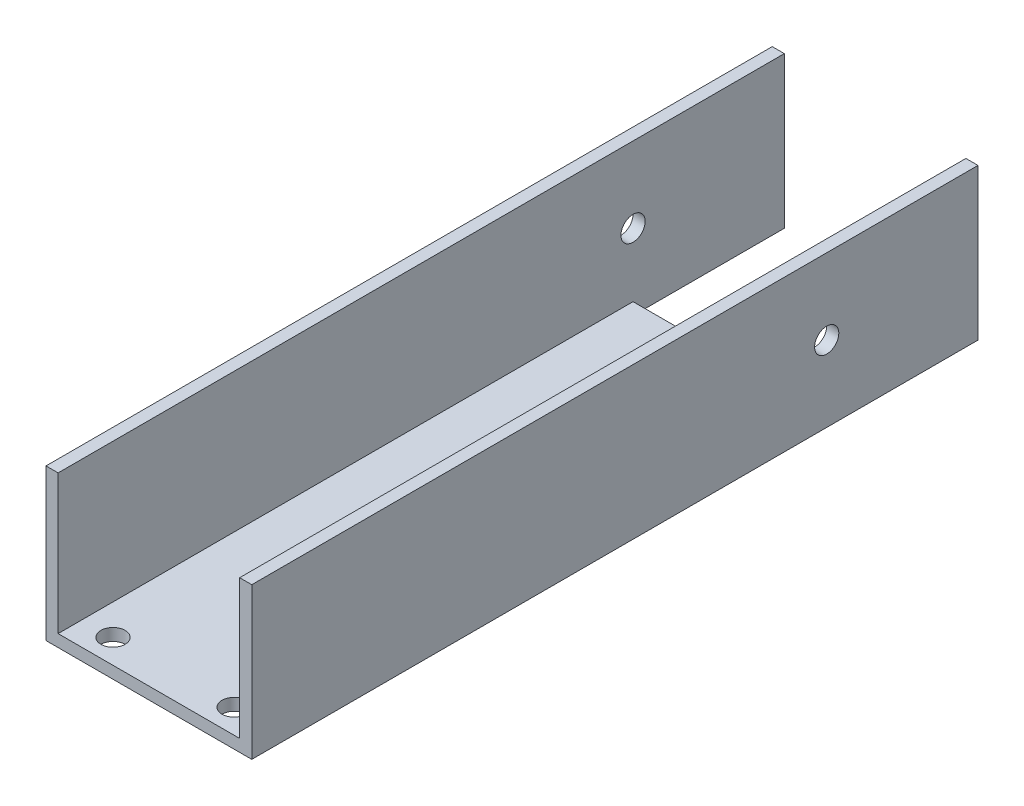
SolidWorks part; units mm, degrees
ref_plane "Front Plane" through (0, 0, 0) normal (0, 0, 1) x (1, 0, 0)
ref_plane "Top Plane" through (0, 0, 0) normal (0, 1, 0) x (1, 0, 0)
ref_plane "Right Plane" through (0, 0, 0) normal (1, 0, 0) x (0, 0, -1)
sketch "Sketch1" plane through (0, 0, 0) normal (0, 0, 1) x (1, 0, 0)
  line L0 (-15, 23) -> (-15, 0)
  line L1 (-15, 0) -> (15, 0)
  line L2 (15, 0) -> (15, 23)
  line L3 (15, 23) -> (17, 23)
  line L4 (17, 23) -> (17, -2)
  line L5 (17, -2) -> (-17, -2)
  line L6 (-17, -2) -> (-17, 23)
  line L7 (-17, 23) -> (-15, 23)
  dimension "D1" = 2
  dimension "D2" = 2
  dimension "D3" = 2
  dimension "D4" = 34
  dimension "D5" = 17
  dimension "D6" = 25
  dimension "D7" = 25
extrude "Boss-Extrude1" add sketch "Sketch1" along normal blind 120
sketch "Sketch2" plane through (0, -2, 0) normal (0, -1, 0) x (1, 0, 0)
  line L0 (-9.9287, 116) -> (0.0713, 98.6795) construction
  line L1 (-9.9287, 116) -> (10.0713, 116) construction
  line L2 (10.0713, 116) -> (9.6327, 114.0487) construction
  line L3 (0.0713, 98.6795) -> (10.0713, 116) construction
  line L4 (-17, 120) -> (17, 120) construction
  line L5 (-9.3219, 114.0943) -> (-9.9287, 116) construction
  line L6 (0.0909, 116) -> (-0.0581, -15.3671) construction
  circle A0 centre (0.0713, 98.6795) radius 2
  circle A1 centre (10.0713, 116) radius 2
  circle A2 centre (-9.9287, 116) radius 2
  dimension "D4" = 4
  dimension "D5" = 4
  dimension "D6" = 4
  dimension "D1" = 60
  dimension "D2" = 60
  dimension "D3" = 20
  dimension "D7" = 4
extrude "Cut-Extrude1" cut sketch "Sketch2" against normal through all
sketch "Sketch3" plane through (0, 0, 0) normal (0, 1, 0) x (1, 0, 0)
  line L0 (15, -120) -> (15, 0) construction
  line L1 (-15, 0) -> (15, 0)
  line L2 (-15, 0) -> (-15, -25)
  line L3 (-15, -25) -> (15, -25)
  line L4 (15, 0) -> (15, -25)
  dimension "D1" = 25
extrude "Cut-Extrude2" cut sketch "Sketch3" against normal through all
sketch "Sketch4" plane through (17, 0, 0) normal (1, 0, 0) x (0, 0, -1)
  line L0 (0, -2) -> (0, 23) construction
  circle A0 centre (-25, 10.5) radius 2
  dimension "D1" = 4
  dimension "D2" = 25
extrude "Cut-Extrude3" cut sketch "Sketch4" against normal through all
